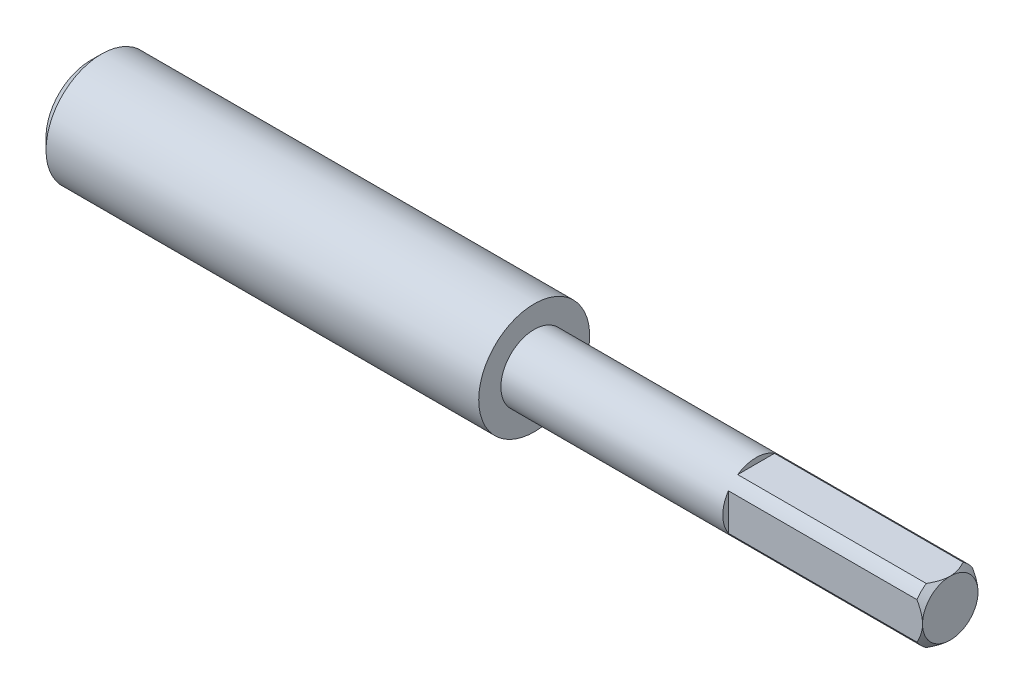
SolidWorks part; units mm, degrees
ref_plane "Front Plane" through (0, 0, 0) normal (0, 0, 1) x (1, 0, 0)
ref_plane "Top Plane" through (0, 0, 0) normal (0, 1, 0) x (1, 0, 0)
ref_plane "Right Plane" through (0, 0, 0) normal (1, 0, 0) x (0, 0, -1)
sketch "Sketch1" plane through (0, 0, 0) normal (0, 0, 1) x (1, 0, 0)
  line L0 (0, 0) -> (0, 10)
  line L1 (0, 10) -> (80, 10)
  line L2 (80, 10) -> (80, 6)
  line L3 (80, 6) -> (155, 6)
  line L4 (155, 6) -> (155, 0)
  line L5 (0, 0) -> (155, 0) construction
  line L6 (0, 0) -> (155, 0)
  dimension "D1" = 6
  dimension "D2" = 10
  dimension "D3" = 75
  dimension "D4" = 80
revolve "Revolve1" add sketch "Sketch1" angle 360 about L6
cosmetic thread "Cosmetic Thread1" parameters "D1"=40, "D2"=10.344
cosmetic thread "Cosmetic Thread2" parameters "D1"=250, "D2"=17.252
chamfer "Chamfer1" distance 1 angle 45 1 edges at (155, 0, 6)
chamfer "Chamfer2" distance 2 angle 45 1 edges at (0, 0, 10)
sketch "Sketch2" plane through (155, 0, 0) normal (1, 0, 0) x (0, 0, -1)
  line L1 (-5, -5) -> (5, -5)
  line L2 (-5, -5) -> (-5, 5)
  line L3 (-5, 5) -> (5, 5)
  line L4 (5, -5) -> (5, 5)
  line L5 (-5, -5) -> (5, 5) construction
  line L6 (-5, 5) -> (5, -5) construction
  point P0 (0, 0)
  dimension "D1" = 10
  dimension "D2" = 10
extrude "Cut-Extrude1" cut sketch "Sketch2" against normal blind 35 flip side to cut
sketch "Sketch3" plane through (0, 0, 0) normal (-1, 0, 0) x (0, 0, 1)
  circle A0 centre (0, 0) radius 8.75
  dimension "D1" = 17.5
